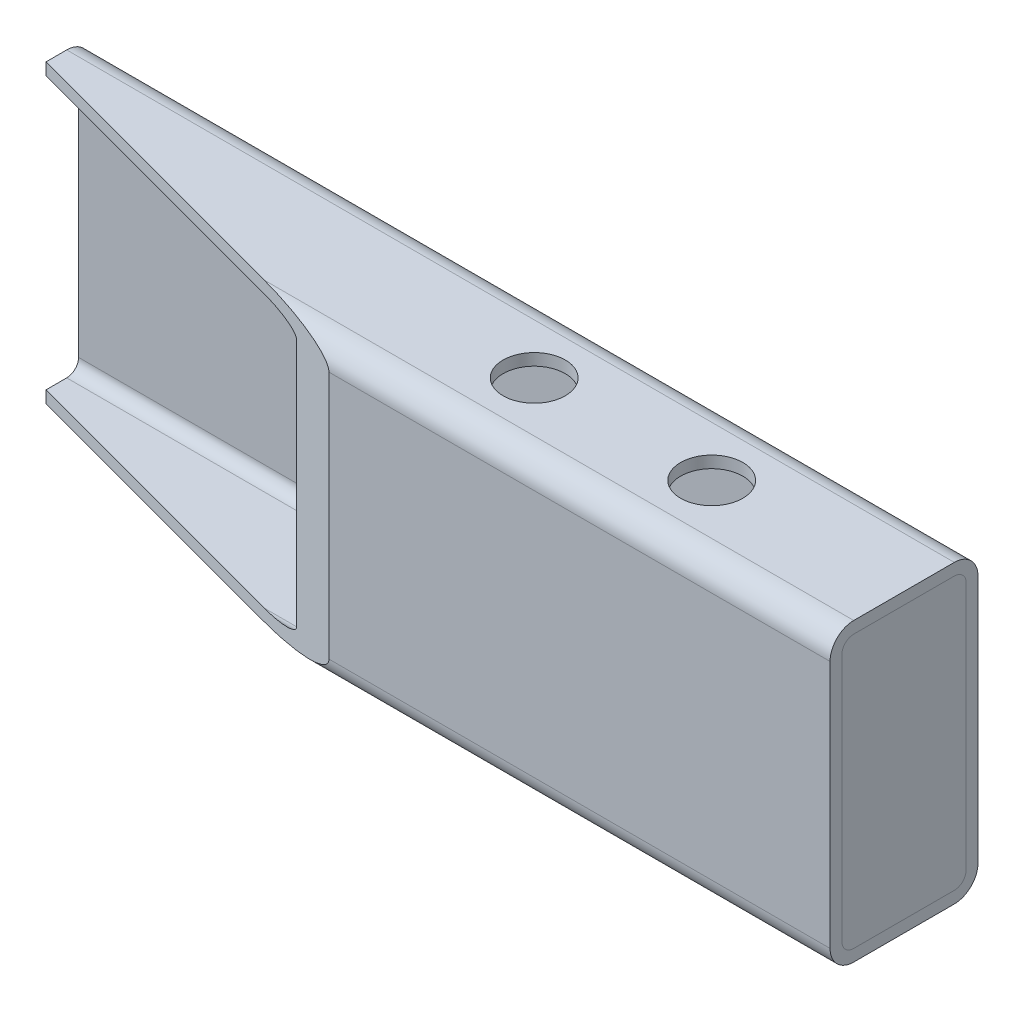
SolidWorks part; units mm, degrees
material "普通碳钢"
ref_plane "Front Plane" through (0, 0, 0) normal (0, 0, 1) x (1, 0, 0)
ref_plane "Top Plane" through (0, 0, 0) normal (0, 1, 0) x (1, 0, 0)
ref_plane "Right Plane" through (0, 0, 0) normal (1, 0, 0) x (0, 0, -1)
sketch3d "3DSketch1"
  line L0 (0, 0, 0) -> (300, 0, 0)
  dimension "D1" = 300
other "Rectangular tube 100 X 50 X 4 (1)"
ref_plane "Plane1" through (0, 0, 0) normal (1, 0, 0) x (0, 0, -1)
sketch "Sketch1" plane through (0, 0, 0) normal (1, 0, 0) x (0, 0, -1)
  line L0 (-17, -46) -> (17, -46)
  line L1 (-21, -42) -> (-21, 42)
  line L2 (17, 46) -> (-17, 46)
  line L3 (21, 42) -> (21, -42)
  line L4 (-17, -50) -> (17, -50)
  line L5 (-25, -42) -> (-25, 42)
  line L6 (17, 50) -> (-17, 50)
  line L7 (25, 42) -> (25, -42)
  arc A0 (25, 42) -> (17, 50) centre (17, 42) ccw
  arc A1 (17, -50) -> (25, -42) centre (17, -42) ccw
  arc A2 (-25, -42) -> (-17, -50) centre (-17, -42) ccw
  arc A3 (-17, 50) -> (-25, 42) centre (-17, 42) ccw
  arc A4 (-17, 46) -> (-21, 42) centre (-17, 42) ccw
  arc A5 (21, 42) -> (17, 46) centre (17, 42) ccw
  arc A6 (17, -46) -> (21, -42) centre (17, -42) ccw
  arc A7 (-21, -42) -> (-17, -46) centre (-17, -42) ccw
  point P0 (0, 50)
  point P1 (25, 0)
  point P2 (0, -50)
  point P3 (-25, 0)
  point P4 (-25, 50)
  point P5 (25, 50)
  point P6 (25, -50)
  point P7 (-25, -50)
  point P8 (0, 0)
  point P33 (0, 0)
  dimension "D1" = 8
  dimension "Thickness" = 4
  dimension "V_leg" = 100
  dimension "H_leg" = 50
sketch "Sketch2" plane through (0, -50, 0) normal (0, -1, 0) x (1, 0, 0)
  line L0 (0, -10) -> (130.6218, 25)
  line L1 (0, 17) -> (0, -17) construction
  line L2 (300, 25) -> (0, 25) construction
  line L3 (130.6218, 25) -> (0, 25)
  line L4 (0, 25) -> (0, -10)
  line L5 (300, 0) -> (0, 0) construction
  line L6 (300, 17) -> (300, -17) construction
  circle A0 centre (235, 0) radius 10.5
  circle A1 centre (175, 0) radius 10.5
  dimension "D3" = 21
  dimension "D4" = 21
  dimension "D1" = 35
  dimension "D2" = 15
  dimension "D5" = 65
  dimension "D6" = 60
extrude "Cut-Extrude1" cut sketch "Sketch2" against normal up to surface (100 mm away) up to face at (150, 50, 0)
sketch "Sketch3" plane through (300, 0, 0) normal (1, 0, 0) x (0, 0, -1)
  line L0 (17, 46) -> (-17, 46) construction
  line L1 (-17, 46) -> (17, 46)
  line L2 (-21, 42) -> (-21, -42)
  line L3 (-17, -46) -> (17, -46)
  line L4 (21, 42) -> (21, -42)
  line L5 (21, -42) -> (21, 42) construction
  line L6 (-21, 42) -> (-21, -42) construction
  line L7 (-17, -46) -> (17, -46) construction
  arc A1 (-21, -42) -> (-17, -46) centre (-17, -42) ccw
  arc A2 (17, -46) -> (21, -42) centre (17, -42) ccw
  arc A3 (17, 46) -> (21, 42) centre (17, 42) cw
  arc A4 (-17, 46) -> (-21, 42) centre (-17, 42) ccw
  dimension "D1" = 4
extrude "Boss-Extrude1" add sketch "Sketch3" against normal blind 25 separate body
